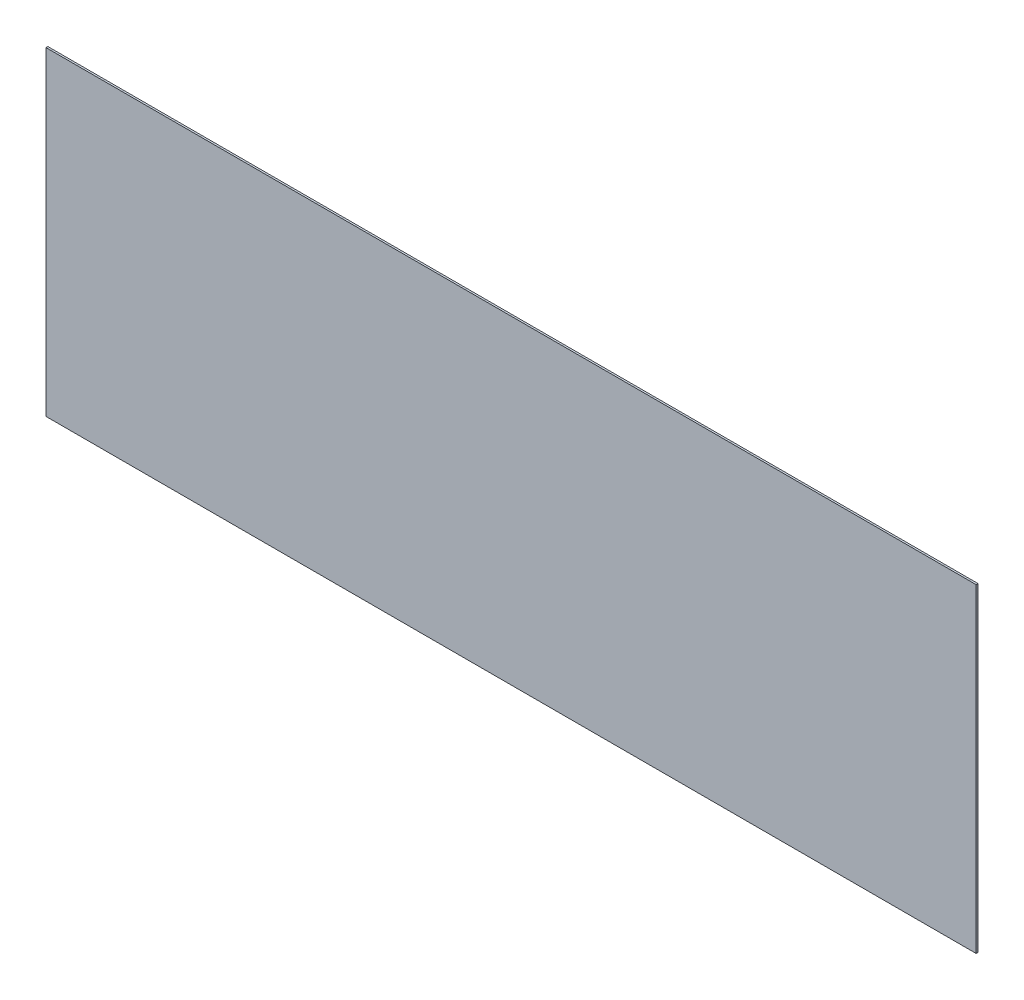
from build123d import *

# Parameters (mm, degrees)
SKETCH_1_W      = 990
SKETCH_1_H      = 340
EXTRUDE_1_DEPTH = 2


with BuildPart() as part:
    # 草图1 → 凸台-拉伸1 (new body)
    with BuildSketch(Plane.XY):
        with Locations((208.496503497, 12.482517483)):
            Rectangle(SKETCH_1_W, SKETCH_1_H)
    extrude(amount=EXTRUDE_1_DEPTH)


solid = part.part
